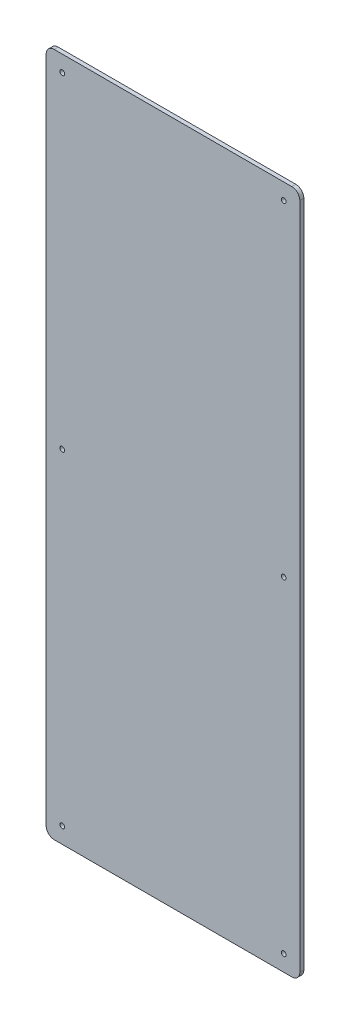
from build123d import *

# Parameters (mm, degrees)
SKETCH_1_W                = 315
SKETCH_1_H                = 850
EXTRUDE_1_DEPTH           = 5
HOLE_WIZARD_6_0_6_1_D     = 6
HOLE_WIZARD_6_0_6_1_DEPTH = 27.75
HOLE_WIZARD_6_0_6_1_TIP   = 1.802581857
FILLET_1_R                = 10


with BuildPart() as part:
    # 草图1 → 凸台-拉伸1 (new body)
    with BuildSketch(Plane.XY):
        Rectangle(SKETCH_1_W, SKETCH_1_H)
    extrude(amount=EXTRUDE_1_DEPTH)

    # Ø6.0 (6) 直径孔1
    with Locations(Plane.XY.offset(5)):
        with Locations((-137.5, 405), (137.5, 405), (137.5, -405), (-137.5, -405), (-137.5, 0), (137.5, 0)):
            Hole(HOLE_WIZARD_6_0_6_1_D / 2, depth=HOLE_WIZARD_6_0_6_1_DEPTH)
            with Locations((0, 0, -(HOLE_WIZARD_6_0_6_1_DEPTH + HOLE_WIZARD_6_0_6_1_TIP / 2))):  # 118° drill point
                Cone(0, HOLE_WIZARD_6_0_6_1_D / 2, HOLE_WIZARD_6_0_6_1_TIP, mode=Mode.SUBTRACT)

    # 圆角1
    fillet_1_edges = [part.edges().sort_by_distance(p)[0] for p in [
        (157.5, -425, 2.5),
        (-157.5, -425, 2.5),
        (-157.5, 425, 2.5),
        (157.5, 425, 2.5),
    ]]
    fillet(fillet_1_edges, radius=FILLET_1_R)


solid = part.part
